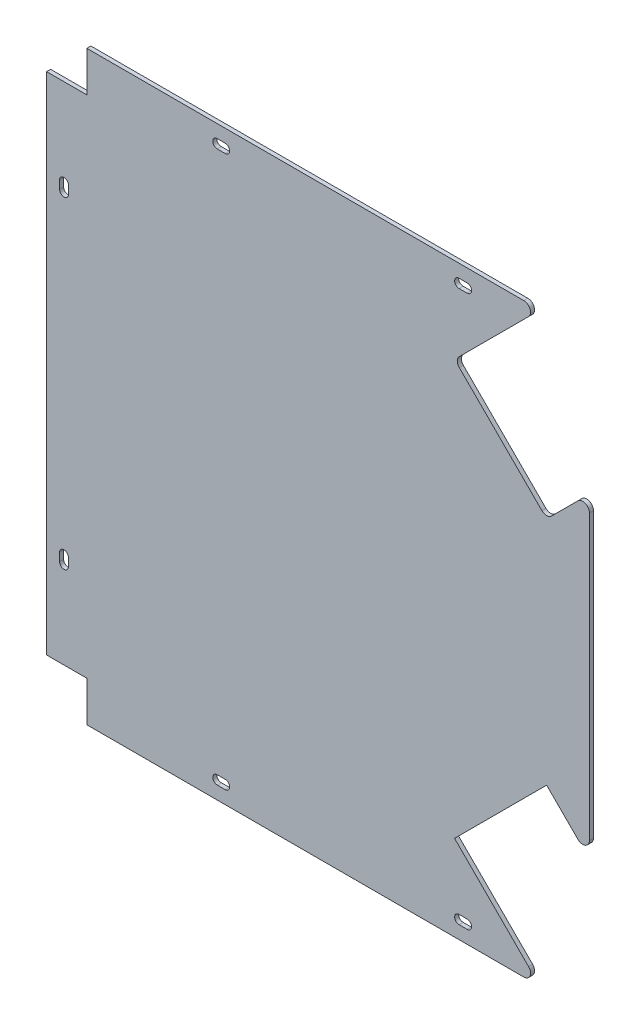
SolidWorks part; units mm, degrees
ref_plane "前视基准面" through (0, 0, 0) normal (0, 0, 1) x (1, 0, 0)
ref_plane "上视基准面" through (0, 0, 0) normal (0, 1, 0) x (1, 0, 0)
ref_plane "右视基准面" through (0, 0, 0) normal (1, 0, 0) x (0, 0, -1)
sketch "草图1" plane through (0, 0, 0) normal (0, 0, 1) x (1, 0, 0)
  line L1 (220, -218) -> (-220, -218)
  line L2 (220, -218) -> (220, 218)
  line L3 (220, 218) -> (-220, 218)
  line L4 (-220, -218) -> (-220, 218)
  line L5 (220, -218) -> (-220, 218) construction
  line L6 (220, 218) -> (-220, -218) construction
  point P0 (0, 0)
  dimension "D1" = 440
  dimension "D2" = 436
extrude "凸台-拉伸1" add sketch "草图1" along normal blind 3
sketch "草图2" plane through (0, 0, 3) normal (0, 0, 1) x (1, 0, 0)
  line L1 (-190, -188) -> (-220, -188)
  line L2 (-190, -188) -> (-190, -218)
  line L3 (-190, -218) -> (-220, -218)
  line L4 (-220, -188) -> (-220, -218)
  line L5 (-190, -188) -> (-220, -218) construction
  line L6 (-190, -218) -> (-220, -188) construction
  line L7 (-190, 188) -> (-220, 188)
  line L8 (-190, 188) -> (-190, 218)
  line L9 (-190, 218) -> (-220, 218)
  line L10 (-220, 188) -> (-220, 218)
  line L11 (-190, 188) -> (-220, 218) construction
  line L12 (-190, 218) -> (-220, 188) construction
  point P0 (-205, -203)
  point P5 (-205, 203)
  dimension "D1" = 30
extrude "切除-拉伸1" cut sketch "草图2" against normal blind 10
sketch "草图3" plane through (0, 0, 3) normal (0, 0, 1) x (1, 0, 0)
  line L0 (20, 218) -> (220, 18)
  line L1 (220, -18) -> (20, -218)
  line L2 (220, 218) -> (-190, 218) construction
  line L3 (220, -218) -> (220, 218) construction
  line L4 (-190, -218) -> (220, -218) construction
  line L13 (-220, -188) -> (-190, -188)
  line L14 (-190, -188) -> (-190, -218)
  line L15 (-190, -218) -> (220, -218)
  line L16 (220, -218) -> (220, 218)
  line L17 (220, 218) -> (-190, 218)
  line L18 (-190, 218) -> (-190, 188)
  line L19 (-190, 188) -> (-220, 188)
  line L20 (-220, 188) -> (-220, -188)
  line L21 (-220, -188) -> (-190, -188)
  line L22 (-190, -188) -> (-190, -218)
  line L23 (-190, -218) -> (220, -218)
  line L24 (220, -218) -> (220, 218)
  line L25 (220, 218) -> (-190, 218)
  line L26 (-190, 218) -> (-190, 188)
  line L27 (-190, 188) -> (-220, 188)
  line L28 (-220, 188) -> (-220, -188)
  line M3 (-190, -218) -> (220, -218)
  line M4 (220, -218) -> (220, 218)
  line M5 (220, 218) -> (-190, 218)
  dimension "D1" = 45
  dimension "D2" = 45
  dimension "D3" = 200
  dimension "D4" = 0
extrude "切除-拉伸2" cut sketch "草图3" against normal blind 10 contours L0 M5 M4 | L1 M4 M3
sketch "草图4" plane through (0, 0, 3) normal (0, 0, 1) x (1, 0, 0)
  line L0 (184, 54) -> (184, -54)
  line L1 (20, 218) -> (220, 18) construction
  line L2 (220, -18) -> (20, -218) construction
  line L13 (220, 18) -> (20, 218)
  line L14 (20, 218) -> (-190, 218)
  line L15 (-190, 218) -> (-190, 188)
  line L16 (-190, 188) -> (-220, 188)
  line L17 (-220, 188) -> (-220, -188)
  line L18 (-220, -188) -> (-190, -188)
  line L19 (-190, -188) -> (-190, -218)
  line L20 (-190, -218) -> (20, -218)
  line L21 (20, -218) -> (220, -18)
  line L22 (220, -18) -> (220, 18)
  line L23 (220, 18) -> (20, 218)
  line L24 (20, 218) -> (-190, 218)
  line L25 (-190, 218) -> (-190, 188)
  line L26 (-190, 188) -> (-220, 188)
  line L27 (-220, 188) -> (-220, -188)
  line L28 (-220, -188) -> (-190, -188)
  line L29 (-190, -188) -> (-190, -218)
  line L30 (-190, -218) -> (20, -218)
  line L31 (20, -218) -> (220, -18)
  line L32 (220, -18) -> (220, 18)
  line M12 (220, 18) -> (20, 218)
  line M20 (20, -218) -> (220, -18)
  line M21 (220, -18) -> (220, 18)
  dimension "D1" = 0
  dimension "D2" = 36
extrude "切除-拉伸3" cut sketch "草图4" against normal blind 10 contours L0 M12 M20 M21
sketch "草图5" plane through (0, 0, 3) normal (0, 0, 1) x (1, 0, 0)
  line L0 (184, 54) -> (184, 117.6396)
  line L1 (184, 117.6396) -> (152.1802, 85.8198)
  line L2 (20, 218) -> (184, 54) construction
  line L3 (20, 218) -> (147.2792, 218)
  line L4 (147.2792, 218) -> (83.6396, 154.3604)
  line L5 (152.1802, 85.8198) -> (184, 54)
  line M4 (184, 54) -> (20, 218)
  dimension "D1" = 90
  dimension "D2" = 45
extrude "凸台-拉伸2" add sketch "草图5" against normal up to surface (3 mm away) contours L4 L3 M4 | L0 L1 M4 up to face at (-79.2, 0, 0)
mirror "镜向1" about plane through (0, 0, 0) normal (0, 1, 0) of "凸台-拉伸2"
fillet "圆角1" radius 5 6 edges at (147.2792, -218, 1.5) (184, -117.6396, 1.5) (83.6396, 154.3604, 1.5) (152.1802, 85.8198, 1.5) (184, 117.6396, 1.5) (147.2792, 218, 1.5)
sketch "草图6" plane through (0, 0, 0) normal (0, 0, -1) x (-1, 0, 0)
  line L16 (-93, 205) -> (-87, 205) construction
  line L17 (-93, 208.3) -> (-87, 208.3)
  line L18 (-93, 201.7) -> (-87, 201.7)
  line L19 (87, 205) -> (93, 205) construction
  line L20 (87, 208.3) -> (93, 208.3)
  line L21 (87, 201.7) -> (93, 201.7)
  line L22 (207, 123) -> (207, 117) construction
  line L23 (210.3, 123) -> (210.3, 117)
  line L24 (203.7, 123) -> (203.7, 117)
  line L25 (207, -117) -> (207, -123) construction
  line L26 (210.3, -117) -> (210.3, -123)
  line L27 (203.7, -117) -> (203.7, -123)
  line L28 (-65.2548, -154.3604) -> (-115.8944, -205)
  line L29 (-115.8944, -205) -> (177, -205)
  line L30 (177, -205) -> (177, -175)
  line L31 (177, -175) -> (207, -175)
  line L32 (207, -175) -> (207, 175)
  line L33 (207, 175) -> (177, 175)
  line L34 (177, 175) -> (177, 205)
  line L35 (177, 205) -> (-115.8944, 205)
  line L36 (-115.8944, 205) -> (-77.9828, 167.0883)
  line L37 (-77.9828, 141.6325) -> (-139.4523, 80.163)
  line L38 (-164.9081, 80.163) -> (-171, 86.2548)
  line L39 (-171, 86.2548) -> (-171, -86.2548)
  line L40 (-171, -86.2548) -> (-152.1802, -67.435)
  line L41 (-152.1802, -67.435) -> (-65.2548, -154.3604)
  line L43 (-115.8944, -205) -> (177, -205) construction
  line L46 (207, -182.5228) -> (207, 175) construction
  line L49 (177, 205) -> (-115.8944, 205) construction
  line L56 (93, -205) -> (87, -205) construction
  line L57 (93, -208.3) -> (87, -208.3)
  line L58 (93, -201.7) -> (87, -201.7)
  line L59 (-93, -205) -> (-87, -205) construction
  line L60 (-93, -201.7) -> (-87, -201.7)
  line L61 (-93, -208.3) -> (-87, -208.3)
  arc A6 (-93, 208.3) -> (-93, 201.7) centre (-93, 205) ccw
  arc A7 (-87, 201.7) -> (-87, 208.3) centre (-87, 205) ccw
  arc A8 (87, 208.3) -> (87, 201.7) centre (87, 205) ccw
  arc A9 (93, 201.7) -> (93, 208.3) centre (93, 205) ccw
  arc A10 (210.3, 123) -> (203.7, 123) centre (207, 123) ccw
  arc A11 (203.7, 117) -> (210.3, 117) centre (207, 117) ccw
  arc A12 (-77.9828, 141.6325) -> (-77.9828, 167.0883) centre (-90.7107, 154.3604) ccw
  arc A13 (-164.9081, 80.163) -> (-139.4523, 80.163) centre (-152.1802, 92.8909) ccw
  arc A16 (210.3, -117) -> (203.7, -117) centre (207, -117) ccw
  arc A17 (203.7, -123) -> (210.3, -123) centre (207, -123) ccw
  arc A18 (93, -208.3) -> (93, -201.7) centre (93, -205) ccw
  arc A19 (87, -201.7) -> (87, -208.3) centre (87, -205) ccw
  arc A20 (-93, -201.7) -> (-93, -208.3) centre (-93, -205) ccw
  arc A21 (-87, -208.3) -> (-87, -201.7) centre (-87, -205) ccw
  point P3 (-90, 205)
  point P8 (90, 205)
  point P18 (207, 120)
  point P26 (207, -120)
  point P35 (90, -205)
  point P44 (-90, -205)
  dimension "D2" = 3.3
  dimension "D3" = 6
  dimension "D4" = 120
  dimension "D5" = 120
  dimension "D6" = 180
  dimension "D7" = 90
  dimension "D8" = 90
  dimension "D9" = 180
  dimension "D1" = 13
extrude "切除-拉伸4" cut sketch "草图6" against normal blind 10
